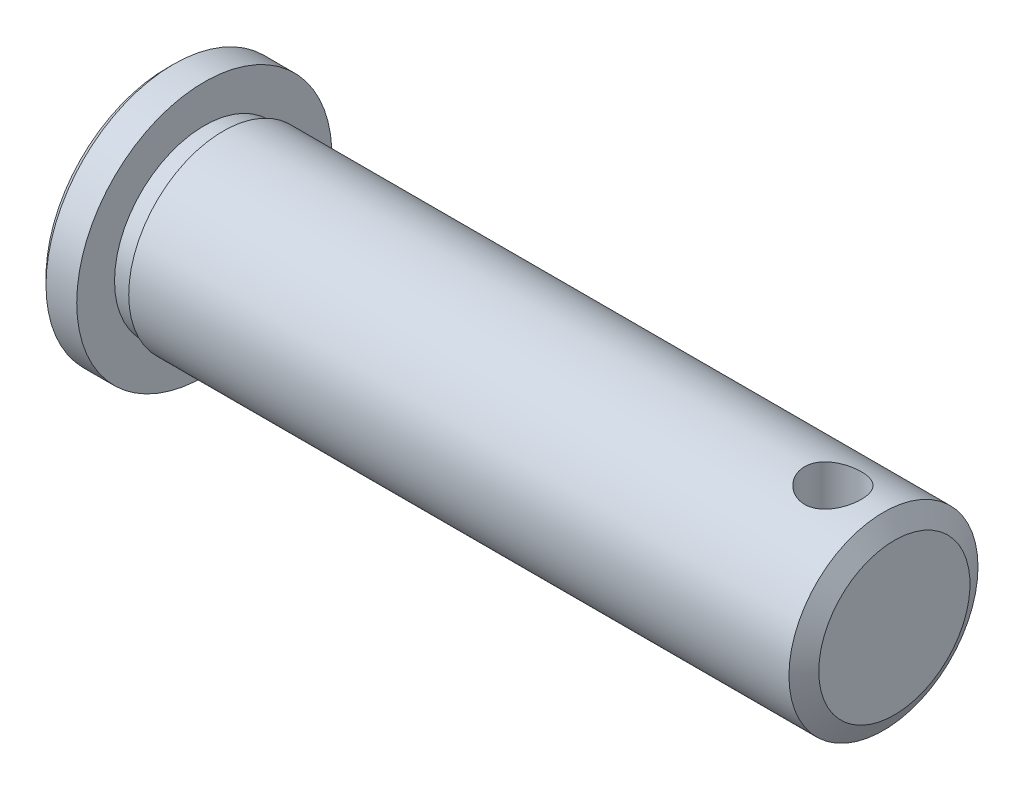
from build123d import *

# Parameters (mm, degrees)
CHAMFER_1_SIZE           = 1.5
CHAMFER_2_SIZE           = 4
CHAMFER_2_SIZE2          = 2.309401077
CUT_EXTRUDE_1_DEPTH      = 159.663165227
CUT_EXTRUDE_1_DEPTH_BACK = 159.663165227
SKETCH_2_R               = 6


with BuildPart() as part:
    # 草图1 → 旋转1 (revolve)
    with BuildSketch(Plane.XY, mode=Mode.PRIVATE) as revolve_1_sk:
        Polygon((0, 0), (154, 0), (154, 20), (12, 20), (12, 19), (8, 19), (8, 27), (0, 27), align=None)
    revolve(revolve_1_sk.sketch.rotate(Axis((-105.652173913, 0, 0), (1, 0, 0)), 90), axis=Axis((-105.652173913, 0, 0), (1, 0, 0)))

    # 倒角1
    chamfer_1_edges = [part.edges().sort_by_distance(p)[0] for p in [
        (0, 0, -27),
    ]]
    chamfer(chamfer_1_edges, length=CHAMFER_1_SIZE)

    # 倒角2
    chamfer_2_edges = [part.edges().sort_by_distance(p)[0] for p in [
        (154, 0, -20),
    ]]
    chamfer_2_side = [part.faces().sort_by_distance(p)[0] for p in [
        (154, 0, 0),
    ]]
    chamfer(chamfer_2_edges, length=CHAMFER_2_SIZE, length2=CHAMFER_2_SIZE2, reference=chamfer_2_side[0])

    # 草图2 → 切除-拉伸1 (cut, two sides: drawn at the far end of the back side and taken through both)
    with BuildSketch(Plane(origin=(0, 0, 0), x_dir=(1, 0, 0), z_dir=(0, 1, 0)).offset(-CUT_EXTRUDE_1_DEPTH_BACK)):
        with Locations(Location((141, 0, 0), (0, 0, 270))):
            Circle(SKETCH_2_R)
    extrude(amount=CUT_EXTRUDE_1_DEPTH + CUT_EXTRUDE_1_DEPTH_BACK, mode=Mode.SUBTRACT)


solid = part.part
